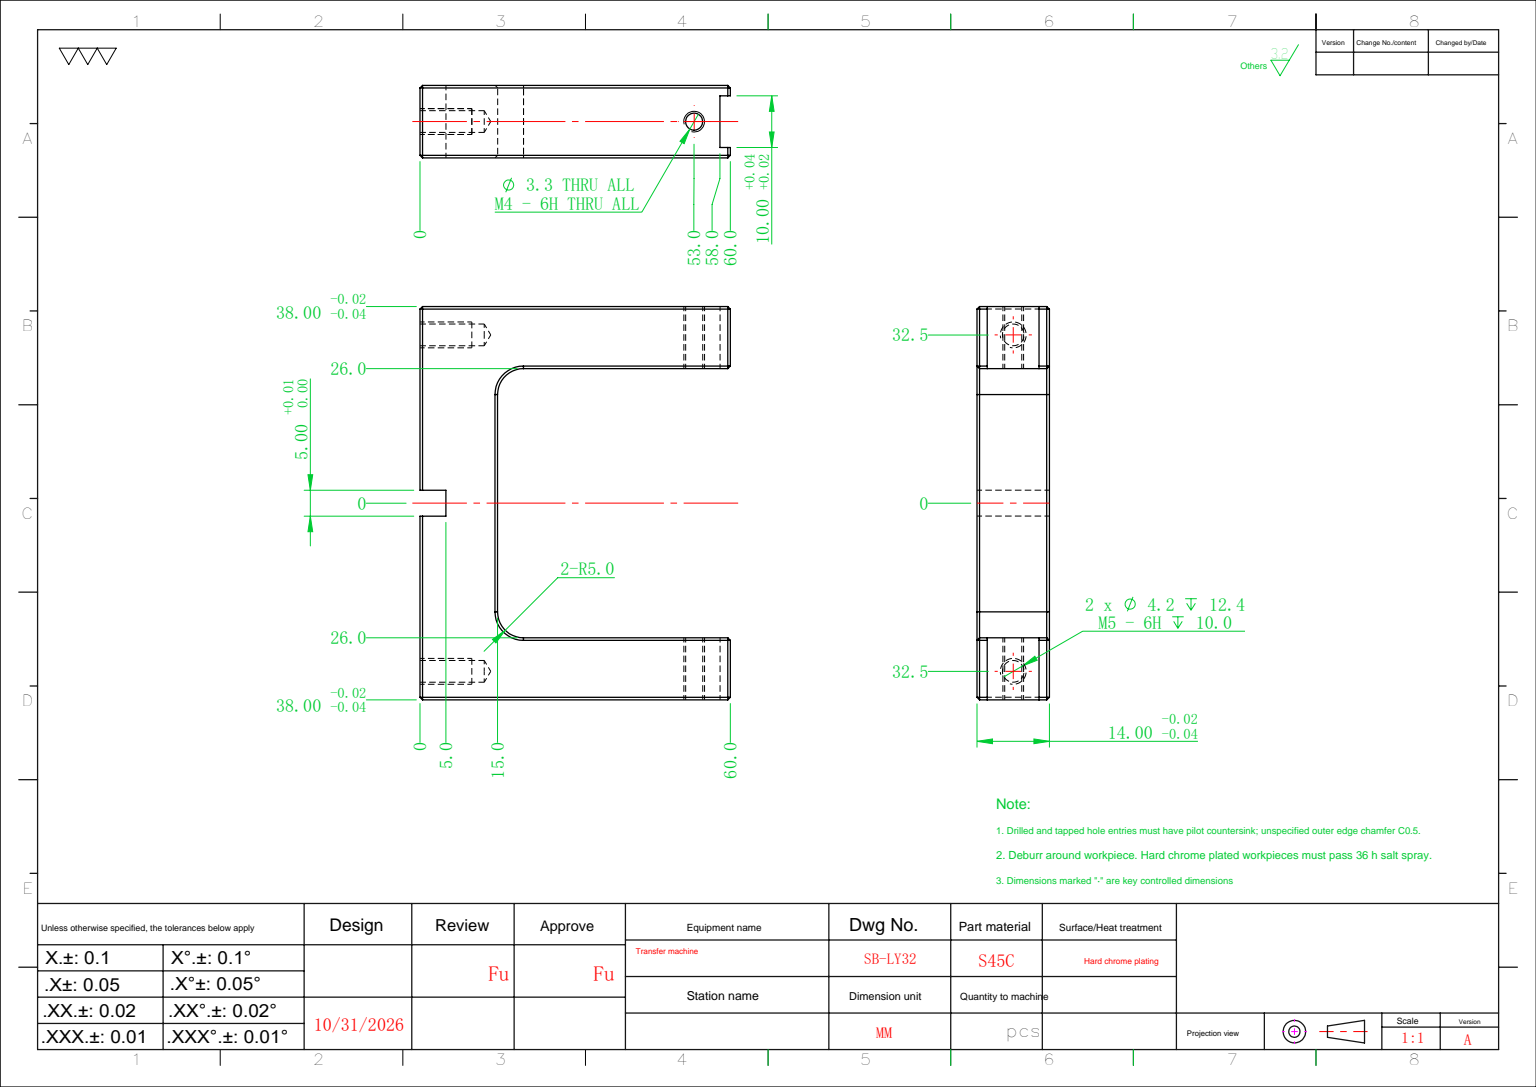
from build123d import *

# Parameters (mm, degrees)
SKETCH_1_W             = 60
SKETCH_1_H             = 76
EXTRUDE_1_DEPTH        = 14
SKETCH_2_W             = 2
SKETCH_2_H             = 10
CUT_EXTRUDE_1_DEPTH    = 83.897527104
SKETCH_3_W             = 45
SKETCH_3_H             = 52
CUT_EXTRUDE_2_DEPTH    = 51.398412673
HOLE_WIZARD_M4_1_D     = 3.3
HOLE_WIZARD_M5_2_D     = 4.2
HOLE_WIZARD_M5_2_DEPTH = 12.4
HOLE_WIZARD_M5_2_TIP   = 1.2618073
SKETCH_8_W             = 5
SKETCH_8_H             = 5
CUT_EXTRUDE_3_DEPTH    = 51.398412673
FILLET_1_R             = 5
CHAMFER_1_SIZE         = 0.5


with BuildPart() as part:
    # 草图1 → 凸台-拉伸1 (new body)
    with BuildSketch(Plane.XY):
        Rectangle(SKETCH_1_W, SKETCH_1_H)
    extrude(amount=EXTRUDE_1_DEPTH)

    # 草图2 → 切除-拉伸1 (cut, through all)
    with BuildSketch(Plane(origin=(0, 38, 0), x_dir=(1, 0, 0), z_dir=(0, 1, 0))):
        with Locations((29, -7)):
            Rectangle(SKETCH_2_W, SKETCH_2_H)
    extrude(amount=-CUT_EXTRUDE_1_DEPTH, mode=Mode.SUBTRACT)

    # 草图3 → 切除-拉伸2 (cut, through all)
    with BuildSketch(Plane(origin=(0, 0, 0), x_dir=(-1, 0, 0), z_dir=(0, 0, -1))):
        with Locations((-7.5, 0)):
            Rectangle(SKETCH_3_W, SKETCH_3_H)
    extrude(amount=-CUT_EXTRUDE_2_DEPTH, mode=Mode.SUBTRACT)

    # M4 螺纹孔1 (through all)
    with Locations(Plane(origin=(0, 38, 0), x_dir=(1, 0, 0), z_dir=(0, 1, 0))):
        with Locations((23, -7)):
            Hole(HOLE_WIZARD_M4_1_D / 2)

    # M5 螺纹孔2
    with Locations(Plane.ZY.offset(30)):
        with Locations((7, 32.5), (7, -32.5)):
            Hole(HOLE_WIZARD_M5_2_D / 2, depth=HOLE_WIZARD_M5_2_DEPTH)
            with Locations((0, 0, -(HOLE_WIZARD_M5_2_DEPTH + HOLE_WIZARD_M5_2_TIP / 2))):  # 118° drill point
                Cone(0, HOLE_WIZARD_M5_2_D / 2, HOLE_WIZARD_M5_2_TIP, mode=Mode.SUBTRACT)

    # 草图8 → 切除-拉伸3 (cut, through all)
    with BuildSketch(Plane.XY.offset(14)):
        with Locations((-27.5, 0)):
            Rectangle(SKETCH_8_W, SKETCH_8_H)
    extrude(amount=-CUT_EXTRUDE_3_DEPTH, mode=Mode.SUBTRACT)

    # 圆角1
    fillet_1_edges = [part.edges().sort_by_distance(p)[0] for p in [
        (-15, -26, 7),
        (-15, 26, 7),
    ]]
    fillet(fillet_1_edges, radius=FILLET_1_R)

    # 倒角1
    chamfer_1_edges = [part.edges().sort_by_distance(p)[0] for p in [
        (-30, 20.25, 14),
        (30, -38, 1),
        (30, 38, 1),
        (0, -38, 14),
        (30, 32, 0),
        (30, 32, 14),
        (30, -26, 13),
        (30, -26, 1),
        (30, 26, 13),
        (30, 26, 1),
        (10, -26, 14),
        (10, -26, 0),
        (30, -32, 14),
        (0, -38, 0),
        (-30, 20.25, 0),
        (0, 38, 0),
        (30, -32, 0),
        (-30, -20.25, 0),
        (-30, -20.25, 14),
        (30, -38, 13),
        (-30, -38, 7),
        (-30, 38, 7),
        (30, 38, 13),
        (0, 38, 14),
        (10, 26, 14),
        (10, 26, 0),
        (-15, 0, 0),
        (-15, 0, 14),
        (-13.535533906, 24.535533906, 0),
        (-13.535533906, 24.535533906, 14),
        (-13.535533906, -24.535533906, 0),
        (-13.535533906, -24.535533906, 14),
    ]]
    chamfer(chamfer_1_edges, length=CHAMFER_1_SIZE)


solid = part.part
